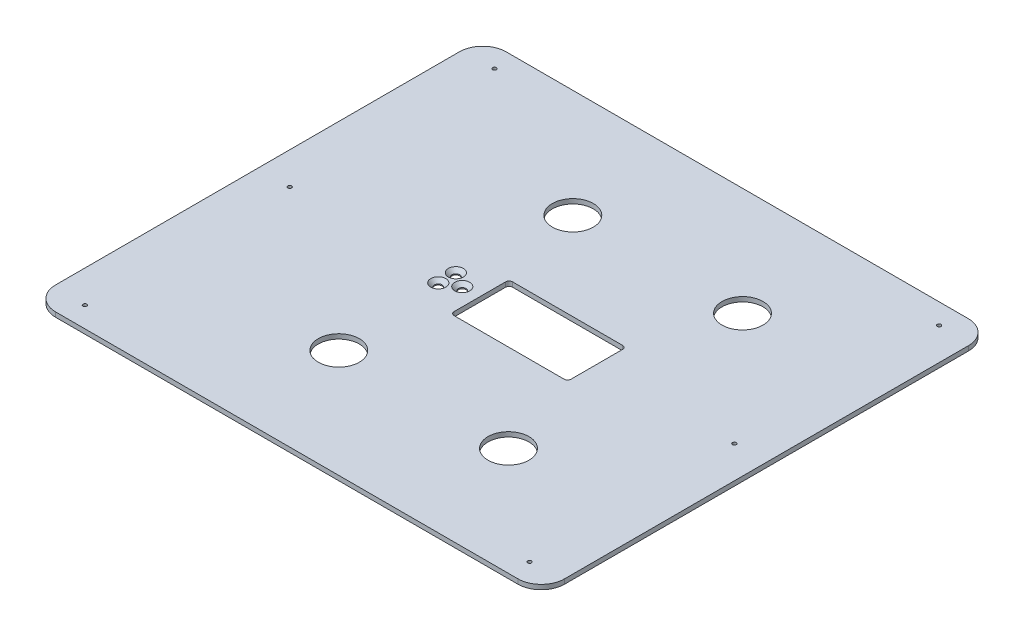
from build123d import *

# Parameters (mm, degrees)
SKETCH1_W                                        = 435
SKETCH1_H                                        = 385
BOSS_EXTRUDE1_DEPTH                              = 4
FILLET1_R                                        = 20
SKETCH2_R                                        = 1.555451355
SKETCH2_R_2                                      = 1.5
SKETCH2_R_3                                      = 1.924870622
CUT_EXTRUDE1_DEPTH                               = 10
CUT_EXTRUDE2_DEPTH                               = 4
HOLE_SIZE_BY_HEXALOBULAR_COUNTERSUNK_D           = 6.6
HOLE_SIZE_BY_HEXALOBULAR_COUNTERSUNK_DEPTH       = 7.5
HOLE_SIZE_BY_HEXALOBULAR_COUNTERSUNK_CSINK_D     = 12.8
HOLE_SIZE_BY_HEXALOBULAR_COUNTERSUNK_CSINK_ANGLE = 90
HOLE_SIZE_BY_HEXALOBULAR_COUNTERSUNK_TIP         = 1.982840043
SKETCH6_R                                        = 17.5
CUT_EXTRUDE3_DEPTH                               = 4
SKETCH7_R                                        = 1.6
CUT_EXTRUDE4_DEPTH                               = 4


with BuildPart() as part:
    # Sketch1 → Boss-Extrude1 (new body)
    with BuildSketch(Plane(origin=(0, 0, 0), x_dir=(1, 0, 0), z_dir=(0, 1, 0))):
        Rectangle(SKETCH1_W, SKETCH1_H)
    extrude(amount=BOSS_EXTRUDE1_DEPTH)

    # Fillet1
    fillet1_edges = [part.edges().sort_by_distance(p)[0] for p in [
        (217.5, 2, 192.5),
        (-217.5, 2, 192.5),
        (-217.5, 2, -192.5),
        (217.5, 2, -192.5),
    ]]
    fillet(fillet1_edges, radius=FILLET1_R)

    # Sketch2 → Cut-Extrude1 (cut)
    with BuildSketch(Plane(origin=(0, 4, 0), x_dir=(1, 0, 0), z_dir=(0, 1, 0))):
        with Locations(Location((-42.5, 0, 0), (0, 0, 270))):
            Circle(SKETCH2_R)
        with Locations(Location((-55.5, 7.5, 0), (0, 0, 270))):
            Circle(SKETCH2_R_2)
        with Locations(Location((-55.5, -7.5, 0), (0, 0, 270))):
            Circle(SKETCH2_R_3)
    extrude(amount=-CUT_EXTRUDE1_DEPTH, mode=Mode.SUBTRACT)

    # Sketch3 → Cut-Extrude2 (cut)
    with BuildSketch(Plane(origin=(0, 4, 0), x_dir=(1, 0, 0), z_dir=(0, 1, 0))):
        with BuildLine():
            Line((-24.5, -25), (69.5, -25))
            ThreePointArc((69.5, -25), (71.621320344, -24.121320344), (72.5, -22))
            Line((72.5, -22), (72.5, 22))
            ThreePointArc((72.5, 22), (71.621320344, 24.121320344), (69.5, 25))
            Line((69.5, 25), (-24.5, 25))
            ThreePointArc((-24.5, 25), (-26.621320344, 24.121320344), (-27.5, 22))
            Line((-27.5, 22), (-27.5, -22))
            ThreePointArc((-27.5, -22), (-26.621320344, -24.121320344), (-24.5, -25))
        make_face()
    extrude(amount=-CUT_EXTRUDE2_DEPTH, mode=Mode.SUBTRACT)

    # Hole Size (% by) Hexalobular Countersunk Head Screw Type1
    with Locations(Plane(origin=(0, 4, 0), x_dir=(1, 0, 0), z_dir=(0, 1, 0))):
        with Locations((-55.5, -7.5), (-42.5, 0), (-55.5, 7.5)):
            CounterSinkHole(HOLE_SIZE_BY_HEXALOBULAR_COUNTERSUNK_D / 2, HOLE_SIZE_BY_HEXALOBULAR_COUNTERSUNK_CSINK_D / 2, depth=HOLE_SIZE_BY_HEXALOBULAR_COUNTERSUNK_DEPTH, counter_sink_angle=HOLE_SIZE_BY_HEXALOBULAR_COUNTERSUNK_CSINK_ANGLE)
            with Locations((0, 0, -(HOLE_SIZE_BY_HEXALOBULAR_COUNTERSUNK_DEPTH + HOLE_SIZE_BY_HEXALOBULAR_COUNTERSUNK_TIP / 2))):  # 118° drill point
                Cone(0, HOLE_SIZE_BY_HEXALOBULAR_COUNTERSUNK_D / 2, HOLE_SIZE_BY_HEXALOBULAR_COUNTERSUNK_TIP, mode=Mode.SUBTRACT)

    # Sketch6 → Cut-Extrude3 (cut)
    with BuildSketch(Plane.XZ):
        with Locations(Location((-48, 100, 0), (0, 0, 270))):
            Circle(SKETCH6_R)
        with Locations(Location((97, 100, 0), (0, 0, 270))):
            Circle(SKETCH6_R)
        with Locations(Location((-48, -100, 0), (0, 0, 270))):
            Circle(SKETCH6_R)
        with Locations(Location((97, -100, 0), (0, 0, 270))):
            Circle(SKETCH6_R)
    extrude(amount=-CUT_EXTRUDE3_DEPTH, mode=Mode.SUBTRACT)

    # Sketch7 → Cut-Extrude4 (cut)
    with BuildSketch(Plane.XZ):
        with Locations(Location((-190, 175, 0), (0, 0, 270))):
            Circle(SKETCH7_R)
        with Locations(Location((-190, 0, 0), (0, 0, 270))):
            Circle(SKETCH7_R)
        with Locations(Location((-190, -175, 0), (0, 0, 270))):
            Circle(SKETCH7_R)
        with Locations(Location((190, 175, 0), (0, 0, 270))):
            Circle(SKETCH7_R)
        with Locations(Location((190, 0, 0), (0, 0, 270))):
            Circle(SKETCH7_R)
        with Locations(Location((190, -175, 0), (0, 0, 270))):
            Circle(SKETCH7_R)
    extrude(amount=-CUT_EXTRUDE4_DEPTH, mode=Mode.SUBTRACT)


solid = part.part
